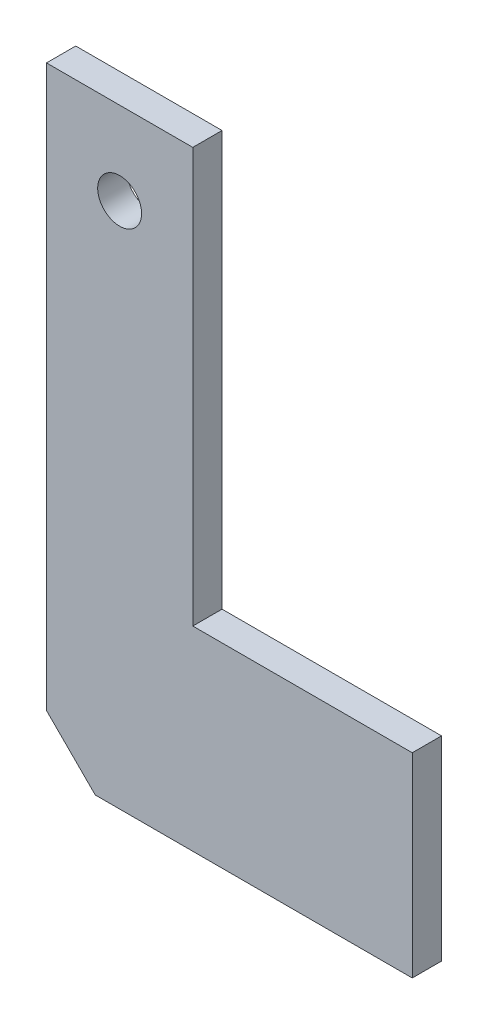
SolidWorks part; units mm, degrees
material "Q235B"
ref_plane "Front" through (0, 0, 0) normal (0, 0, 1) x (1, 0, 0)
ref_plane "Top" through (0, 0, 0) normal (0, 1, 0) x (1, 0, 0)
ref_plane "Right" through (0, 0, 0) normal (1, 0, 0) x (0, 0, -1)
sketch "Sketch1" plane through (0, 0, 0) normal (0, 0, 1) x (1, 0, 0)
  line L0 (-33.5216, -86.6225) -> (-33.5216, 38.3775)
  line L1 (-33.5216, 38.3775) -> (-3.5216, 38.3775)
  line L2 (-3.5216, 38.3775) -> (-3.5216, -46.6225)
  line L3 (-3.5216, -46.6225) -> (41.4784, -46.6225)
  line L4 (41.4784, -46.6225) -> (41.4784, -86.6225)
  line L5 (41.4784, -86.6225) -> (-33.5216, -86.6225)
  dimension "D1" = 75
  dimension "D2" = 125
  dimension "D3" = 30
  dimension "D4" = 40
extrude "Boss-Extrude1" add sketch "Sketch1" along normal blind 6
sketch "Sketch2" plane through (0, 0, 6) normal (0, 0, 1) x (1, 0, 0)
  line L0 (-3.5216, 38.3775) -> (-33.5216, 38.3775) construction
  line L1 (-18.5216, 38.3775) -> (-18.5216, 26.5641) construction
  line L2 (-33.5216, -86.6225) -> (41.4784, -86.6225) construction
  circle A0 centre (-18.5216, 21.3775) radius 4.5
  dimension "D1" = 108
  dimension "D2" = 9
extrude "Cut-Extrude1" cut sketch "Sketch2" against normal up to next
chamfer "Chamfer1" distance 10 angle 45 1 edges at (-33.5216, -86.6225, 3)
equation "\"零件重量\"= IIF ( \"SW-质量\" > 100 , int ( \"SW-质量\" ) , \"SW-质量\" )"
